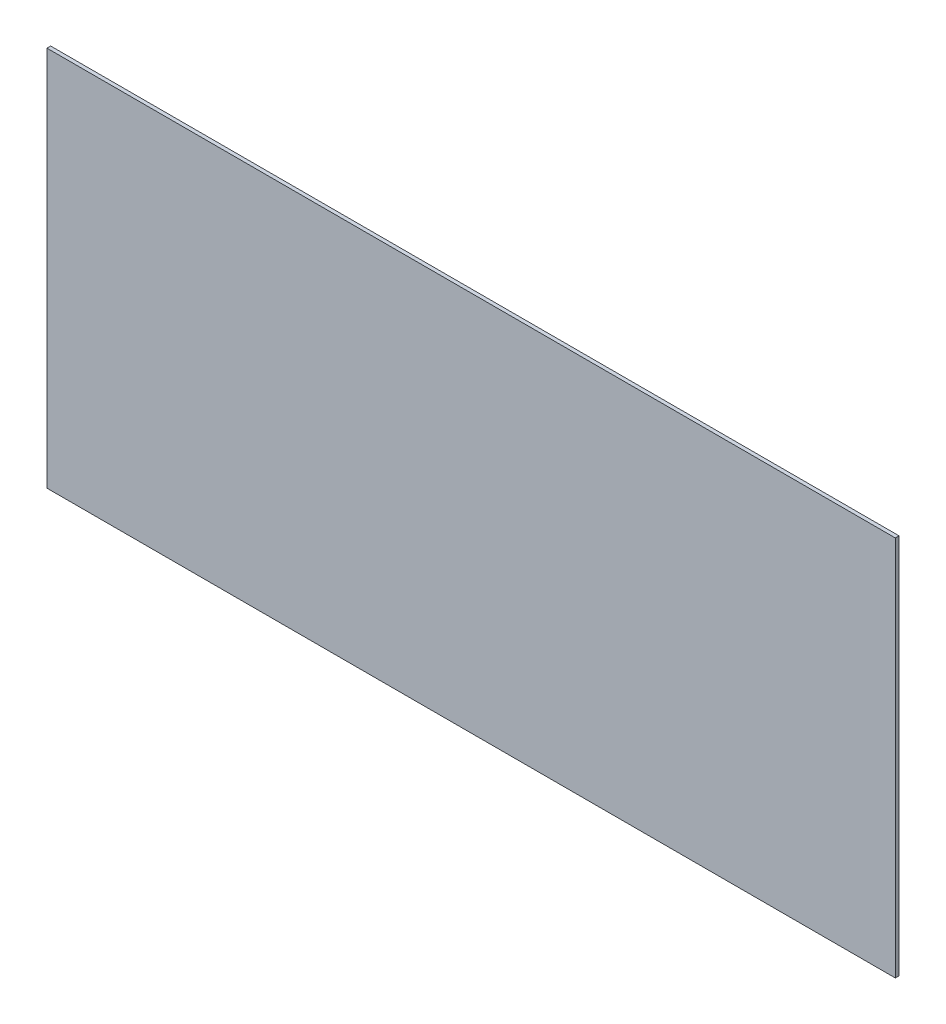
SolidWorks part; units mm, degrees
material "PMMA(有机玻璃)"
ref_plane "前视" through (0, 0, 0) normal (0, 0, 1) x (1, 0, 0)
ref_plane "上视" through (0, 0, 0) normal (0, 1, 0) x (1, 0, 0)
ref_plane "右视" through (0, 0, 0) normal (1, 0, 0) x (0, 0, -1)
sketch "草图1" plane through (0, 0, 0) normal (0, 0, 1) x (1, 0, 0)
  line L1 (-571, 256.5) -> (571, 256.5)
  line L2 (-571, 256.5) -> (-571, -256.5)
  line L3 (-571, -256.5) -> (571, -256.5)
  line L4 (571, 256.5) -> (571, -256.5)
  line L5 (-571, 256.5) -> (571, -256.5) construction
  line L6 (-571, -256.5) -> (571, 256.5) construction
  point P0 (0, 0)
  dimension "D1" = 513
  dimension "D2" = 1142
extrude "凸台-拉伸1" add sketch "草图1" along normal blind 5
hole_wizard "M5 间隙孔1" positions "草图3" profile "草图2" hole size "M5" standard "GB"
sketch "草图3" plane through (0, 0, 5) normal (0, 0, 1) x (1, 0, 0)
  line L0 (-427.5, 273) -> (-427.5, -273) construction
  line L1 (-427.5, -273) -> (427.5, -273) construction
  line L2 (0, 273) -> (0, -273) construction
  line L3 (427.5, 273) -> (-427.5, 273) construction
  line L5 (-427.5, 0) -> (427.5, 0) construction
  line L6 (427.5, -273) -> (427.5, 273) construction
  point P0 (-375, -261)
  point P46 (415.5, 250)
  point P48 (-415.5, 250)
  point P58 (-125, -261)
  point P59 (125, -261)
  point P61 (-125, 261)
  point P62 (125, 261)
  point P64 (-375, 261)
  point P88 (375, -261)
  point P89 (375, 261)
  point P108 (415.5, 0)
  point P109 (-415.5, 0)
  point P110 (415.5, -250)
  point P111 (-415.5, -250)
  dimension "D1" = 12
  dimension "D2" = 12
  dimension "D5" = 3
  dimension "D3" = 12
  dimension "D6" = 4
  dimension "D4" = 2
sketch "草图2" plane through (-375, -261, 5) normal (1, 0, 0) x (0, -1, 0)
  line L0 (0, 0) -> (0, 5)
  line L1 (0, 5) -> (2.75, 5)
  line L2 (2.75, 5) -> (2.75, 0)
  line L5 (2.75, 0) -> (0, 0)
  line L11 (0, -6.35) -> (0, 107.95) construction
  dimension "通孔孔直径" = 5.5
  dimension "通孔孔深度" = 5
